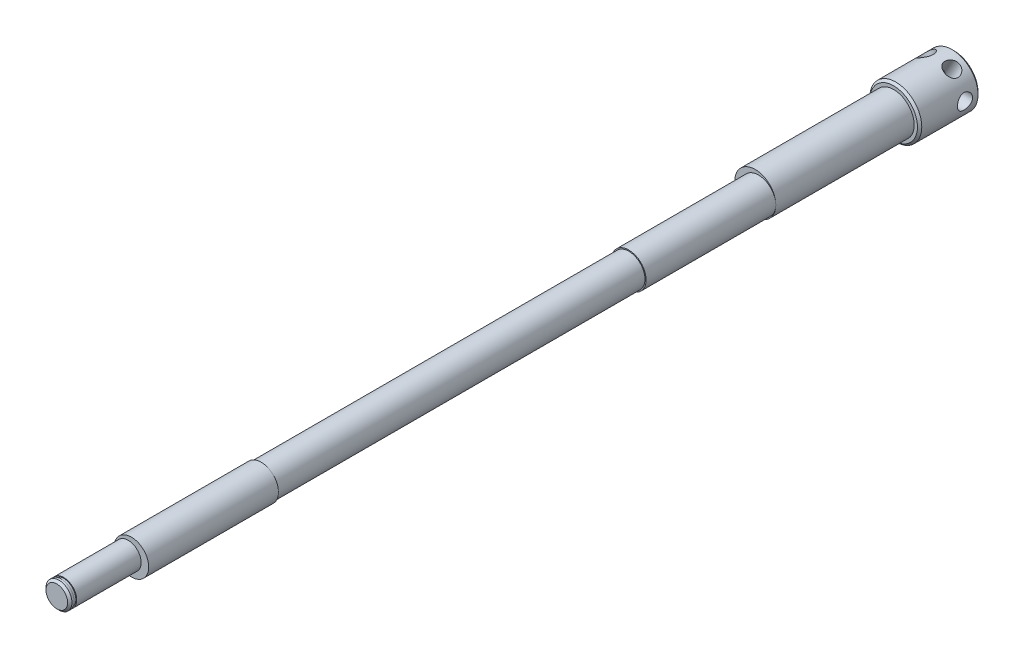
SolidWorks part; units mm, degrees
material "45"
ref_plane "Front Plane" through (0, 0, 0) normal (0, 0, 1) x (1, 0, 0)
ref_plane "Top Plane" through (0, 0, 0) normal (0, 1, 0) x (1, 0, 0)
ref_plane "Right Plane" through (0, 0, 0) normal (1, 0, 0) x (0, 0, -1)
sketch "Sketch1" plane through (0, 0, 0) normal (0, 0, 1) x (1, 0, 0)
  circle A0 centre (0, 0) radius 6
  dimension "D1" = 12
extrude "Boss-Extrude1" add sketch "Sketch1" along normal mid plane 14
sketch "Sketch2" plane through (0, 0, 7) normal (0, 0, 1) x (1, 0, 0)
  circle A0 centre (0, 0) radius 4.75
  dimension "D1" = 9.5
extrude "Boss-Extrude2" add sketch "Sketch2" along normal blind 32
sketch "Sketch3" plane through (0, 0, 39) normal (0, 0, 1) x (1, 0, 0)
  line L0 (0, 0) -> (-0.8489, 0) construction
  circle A0 centre (0.75, 0) radius 4
  dimension "D1" = 0.75
  dimension "D2" = 8
extrude "Boss-Extrude3" add sketch "Sketch3" along normal blind 30
sketch "Sketch4" plane through (0, 0, 69) normal (0, 0, 1) x (1, 0, 0)
  circle A0 centre (0.75, 0) radius 3.75
  circle A1 centre (0.75, 0) radius 4 construction
  dimension "D1" = 7.5
extrude "Boss-Extrude4" add sketch "Sketch4" along normal blind 85
sketch "Sketch5" plane through (0, 0, 154) normal (0, 0, 1) x (1, 0, 0)
  circle A0 centre (0.75, 0) radius 4
  circle A1 centre (0.75, 0) radius 3.75 construction
  dimension "D1" = 8
extrude "Boss-Extrude5" add sketch "Sketch5" along normal blind 30
sketch "Sketch6" plane through (0, 0, 184) normal (0, 0, 1) x (1, 0, 0)
  circle A0 centre (0, 0) radius 3
  circle A1 centre (0, 0) radius 6 construction
  dimension "D1" = 6
extrude "Boss-Extrude6" add sketch "Sketch6" along normal blind 16.5
sketch "Sketch8" plane through (0, 0, 0) normal (0, 1, 0) x (1, 0, 0)
  line L0 (0, 0) -> (0, -223.1532) construction
  line L1 (-3, -200.5) -> (3, -200.5) construction
  line L2 (2.8, -198.9) -> (4.3315, -198.9)
  line L3 (2.8, -198.9) -> (2.8, -199.5)
  line L4 (2.8, -199.5) -> (4.3315, -199.5)
  line L5 (4.3315, -198.9) -> (4.3315, -199.5)
  line L6 (2.8, -198.9) -> (4.3315, -199.5) construction
  line L7 (2.8, -199.5) -> (4.3315, -198.9) construction
  point P3 (3.5657, -199.2)
  dimension "D1" = 0.6
  dimension "D2" = 1
  dimension "D3" = 2.8
revolve "Cut-Revolve1" cut sketch "Sketch8" angle 360 about L0
chamfer "Chamfer1" distance 0.5 angle 45 2 edges at (6, 0, 7) (6, 0, -7)
sketch "Sketch10" plane through (0, 0, 200.5) normal (0, 0, 1) x (1, 0, 0)
  line L0 (0, 0) -> (4.75, 0) construction
  line L1 (4.75, 0) -> (4.75, 6.116) construction
  circle A0 centre (0, 0) radius 4.75 construction
sketch "Sketch11" plane through (0, 0, 0) normal (1, 0, 0) x (0, 0, -1)
  line L0 (0, 0) -> (3.5, 0) construction
  circle A0 centre (3.5, 0) radius 1.75
  dimension "D1" = 3.5
  dimension "D2" = 3.5
extrude "Cut-Extrude1" cut sketch "Sketch11" against normal mid plane 23
pattern_circular "CirPattern1" count 3 every 60 about axis through (0, 0, 7) along (0, 0, -1) of "Cut-Extrude1"
chamfer "Chamfer2" distance 0.5 angle 45 1 edges at (3, 0, 200.5)
